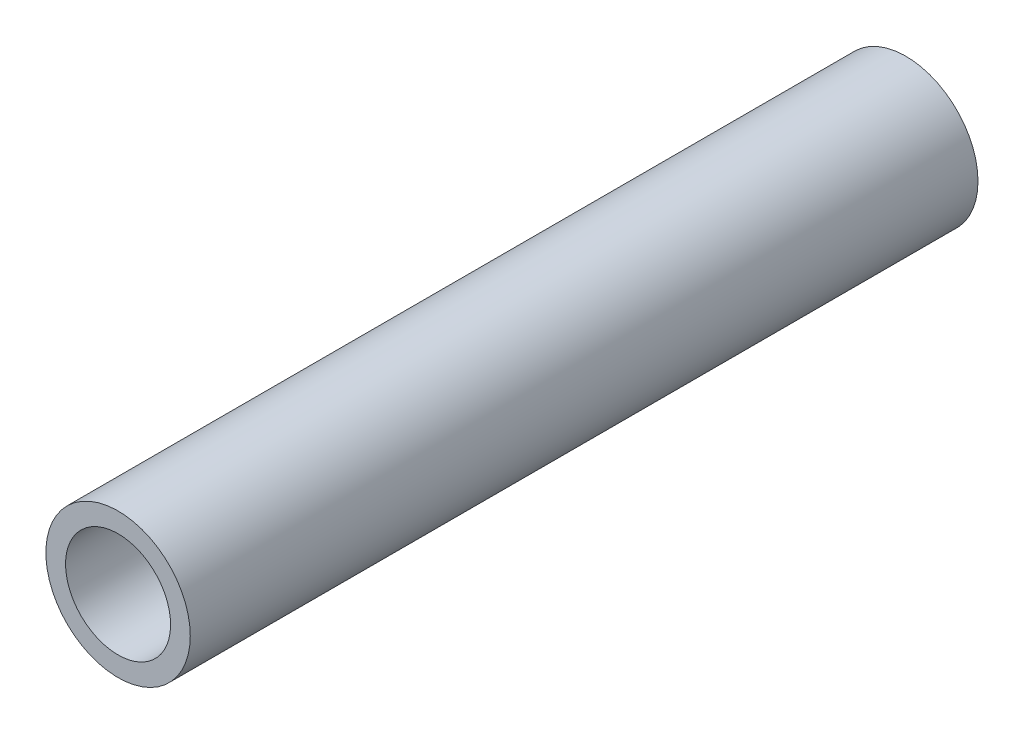
SolidWorks part; units mm, degrees
ref_plane "Front Plane" through (0, 0, 0) normal (0, 0, 1) x (1, 0, 0)
ref_plane "Top Plane" through (0, 0, 0) normal (0, 1, 0) x (1, 0, 0)
ref_plane "Right Plane" through (0, 0, 0) normal (1, 0, 0) x (0, 0, -1)
sketch "Sketch 1" plane through (0, 0, 0) normal (0, 0, 1) x (1, 0, 0)
  circle A0 centre (0, 0) radius 11
  circle A1 centre (0, 0) radius 8
  dimension "D1" = 22
  dimension "D2" = 3
extrude "Boss-Extrude 1" add sketch "Sketch 1" along normal blind 120
